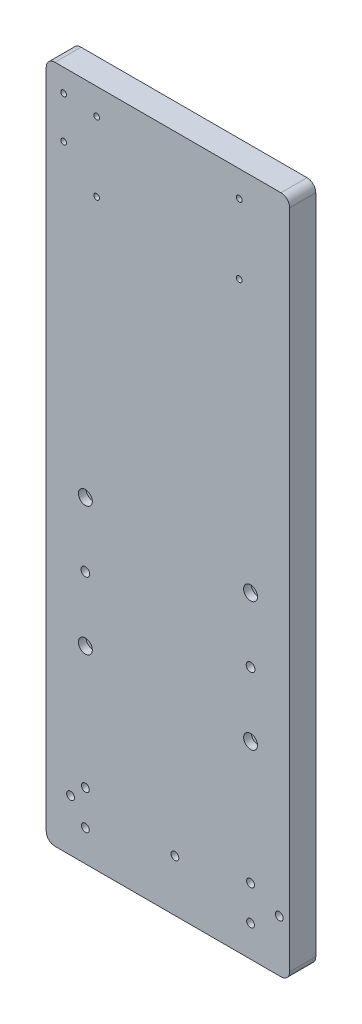
SolidWorks part; units mm, degrees
ref_plane "前视基准面" through (0, 0, 0) normal (0, 0, 1) x (1, 0, 0)
ref_plane "上视基准面" through (0, 0, 0) normal (0, 1, 0) x (1, 0, 0)
ref_plane "右视基准面" through (0, 0, 0) normal (1, 0, 0) x (0, 0, -1)
sketch "草图1" plane through (0, 0, 0) normal (0, 0, 1) x (1, 0, 0)
  line L1 (-70, 195.25) -> (70, 195.25)
  line L2 (-70, 195.25) -> (-70, -195.25)
  line L3 (-70, -195.25) -> (70, -195.25)
  line L4 (70, 195.25) -> (70, -195.25)
  line L5 (-70, 195.25) -> (70, -195.25) construction
  line L6 (-70, -195.25) -> (70, 195.25) construction
  point P0 (0, 0)
  dimension "D1" = 140
  dimension "D2" = 390.5
extrude "凸台-拉伸1" add sketch "草图1" along normal blind 15
sketch "草图29" plane through (0, 0, 0) normal (0, 0, -1) x (-1, 0, 0)
  line L0 (0, 0) -> (-70, 0) construction
  line L1 (-7.5, 45) -> (7.5, 45)
  line L2 (-7.5, 45) -> (-7.5, -45)
  line L3 (-7.5, -45) -> (7.5, -45)
  line L4 (7.5, 45) -> (7.5, -45)
  line L5 (-70, 195.25) -> (70, 195.25) construction
  line L10 (-70, -195.25) -> (-70, 195.25) construction
  line L11 (0, 195.25) -> (0, 0) construction
  dimension "D2" = 90
  dimension "D4" = 15
extrude "凸台-拉伸6" [suppressed] add sketch "草图29" against normal blind 165
hole_wizard "M5 六角凹头螺钉的柱形沉头孔6" positions "草图30" profile "草图31" counterbore size "M4" standard "ISO" end condition through all
sketch "草图30" plane through (0, 0, 15) normal (0, 0, 1) x (1, 0, 0)
  circle A0 centre (47.5, -12.75) radius 2.1 construction
  circle A1 centre (-47.5, -12.75) radius 2.1 construction
  circle A2 centre (47.5, -86.75) radius 2.1 construction
  circle A3 centre (-47.5, -86.75) radius 2.1 construction
  point P0 (-47.5, -12.75)
  point P4 (-47.5, -86.75)
  point P6 (47.5, -12.75)
  point P10 (47.5, -86.75)
sketch "草图31" plane through (-47.5, -12.75, 15) normal (1, 0, 0) x (0, -1, 0)
  line L0 (0, 0) -> (0, 15)
  line L1 (0, 15) -> (2.25, 15)
  line L3 (2.25, 15) -> (2.25, 4.4)
  line L4 (2.25, 4.4) -> (4, 4.4)
  line L5 (4, 4.4) -> (4, 0)
  line L7 (4, 0) -> (0, 0)
  line L11 (0, -6.35) -> (0, 107.95) construction
  dimension "通孔孔直径" = 4.5
  dimension "通孔孔深度" = 15
  dimension "柱形沉头孔直径" = 8
  dimension "柱形沉头孔深度" = 4.4
hole_wizard "Ø5.0 (5) 直径孔1" positions "草图32" profile "草图33" hole size "Ø5.0" standard "ISO" end condition through all
sketch "草图32" plane through (0, 0, 15) normal (0, 0, 1) x (1, 0, 0)
  circle A0 centre (47.5, -49.75) radius 2.5 construction
  circle A1 centre (-47.5, -49.75) radius 2.5 construction
  point P0 (-47.5, -49.75)
  point P2 (47.5, -49.75)
sketch "草图33" plane through (-47.5, -49.75, 15) normal (1, 0, 0) x (0, -1, 0)
  line L0 (0, 0) -> (0, 15)
  line L1 (0, 15) -> (2.5, 15)
  line L2 (2.5, 15) -> (2.5, 0)
  line L5 (2.5, 0) -> (0, 0)
  line L11 (0, -6.35) -> (0, 107.95) construction
  dimension "通孔孔直径" = 5
  dimension "通孔孔深度" = 15
fillet "圆角1" radius 5 4 edges at (70, -195.25, 7.5) (70, 195.25, 7.5) (-70, -195.25, 7.5) (-70, 195.25, 7.5)
hole_wizard "M4 螺纹孔3" positions "草图38" profile "草图39" tap size "M4" standard "ISO" end condition through all
sketch "草图38" plane through (0, 0, 15) normal (0, 0, 1) x (1, 0, 0)
  point P0 (-41, 180.25)
  point P3 (41, 180.25)
  point P6 (41, 140.25)
  point P9 (-41, 140.25)
sketch "草图39" plane through (-41, 180.25, 15) normal (1, 0, 0) x (0, -1, 0)
  line L0 (0, 0) -> (0, 15)
  line L1 (0, 15) -> (1.65, 15)
  line L2 (1.65, 15) -> (1.65, 0)
  line L5 (1.65, 0) -> (0, 0)
  line L11 (0, -6.35) -> (0, 107.95) construction
  dimension "通孔螺纹孔钻头直径" = 3.3
  dimension "通孔螺纹孔钻头深度" = 15
cosmetic thread "孔螺蚊线8" parameters "D2"=4
cosmetic thread "孔螺蚊线9" parameters "D2"=4
cosmetic thread "孔螺蚊线23" parameters "D2"=4
cosmetic thread "孔螺蚊线24" parameters "D2"=4
hole_wizard "M4 六角凹头螺钉的柱形沉头孔1" positions "草图44" profile "草图45" counterbore size "M4" standard "ISO" end condition through all
sketch "草图44" plane through (0, 0, 0) normal (0, 0, -1) x (-1, 0, 0)
  circle A0 centre (47.5, -157.25) radius 1.65 construction
  circle A1 centre (47.5, -177.25) radius 1.65 construction
  circle A2 centre (-47.5, -157.25) radius 1.65 construction
  circle A3 centre (-47.5, -177.25) radius 1.65 construction
  point P0 (47.5, -157.25)
  point P2 (47.5, -177.25)
  point P4 (-47.5, -157.25)
  point P6 (-47.5, -177.25)
sketch "草图45" plane through (-47.5, -157.25, 0) normal (1, 0, 0) x (0, 1, 0)
  line L0 (0, 0) -> (0, 15)
  line L1 (0, 15) -> (2.25, 15)
  line L3 (2.25, 15) -> (2.25, 4.4)
  line L4 (2.25, 4.4) -> (4, 4.4)
  line L5 (4, 4.4) -> (4, 0)
  line L7 (4, 0) -> (0, 0)
  line L11 (0, -6.35) -> (0, 107.95) construction
  dimension "通孔孔直径" = 4.5
  dimension "通孔孔深度" = 15
  dimension "柱形沉头孔直径" = 8
  dimension "柱形沉头孔深度" = 4.4
hole_wizard "M4 螺纹孔6" positions "草图48" profile "草图50" tap size "M4" standard "ISO"
sketch "草图48" plane through (-70, 0, 0) normal (-1, 0, 0) x (0, 0, 1)
  line L0 (7.5, 195.25) -> (7.5, -195.25) construction
  line L1 (0, 195.25) -> (15, 195.25) construction
  line L2 (15, -195.25) -> (0, -195.25) construction
  point P0 (7.5, 185.25)
  point P2 (7.5, 170.25)
  point P4 (7.5, 155.25)
  dimension "D1" = 10
  dimension "D2" = 15
  dimension "D3" = 15
sketch "草图50" plane through (-70, 185.25, 7.5) normal (0, 1, 0) x (0, 0, 1)
  line L0 (0, 0) -> (0, 15.9914)
  line L1 (0, 15.9914) -> (1.65, 15)
  line L2 (1.65, 15) -> (1.65, 0)
  line L5 (1.65, 0) -> (0, 0)
  line L10 (0, 15.9914) -> (-1.65, 15) construction
  line L11 (0, -6.35) -> (0, 107.95) construction
  dimension "螺纹孔钻头直径" = 3.3
  dimension "螺纹孔钻头深度" = 15
  dimension "导头角度" = 118
cosmetic thread "孔螺蚊线18" parameters "D1"=15, "D2"=4
cosmetic thread "孔螺蚊线19" parameters "D1"=15, "D2"=4
cosmetic thread "孔螺蚊线20" parameters "D1"=15, "D2"=4
hole_wizard "M4 螺纹孔7" positions "草图51" profile "草图52" tap size "M4" standard "ISO" end condition through all
sketch "草图51" plane through (0, 0, 15) normal (0, 0, 1) x (1, 0, 0)
  line L0 (-60, 190.25) -> (-60, 150.25)
  arc A0 (-57.75, 188) -> (-62.25, 188) centre (-60, 188) ccw construction
  arc A1 (-62.25, 152.5) -> (-57.75, 152.5) centre (-60, 152.5) ccw construction
  point P0 (-60, 182.25)
  point P2 (-60, 158.25)
  dimension "D1" = 8
  dimension "D2" = 8
sketch "草图52" plane through (-60, 182.25, 15) normal (1, 0, 0) x (0, -1, 0)
  line L0 (0, 0) -> (0, 15)
  line L1 (0, 15) -> (1.65, 15)
  line L2 (1.65, 15) -> (1.65, 0)
  line L5 (1.65, 0) -> (0, 0)
  line L11 (0, -6.35) -> (0, 107.95) construction
  dimension "通孔螺纹孔钻头直径" = 3.3
  dimension "通孔螺纹孔钻头深度" = 15
cosmetic thread "孔螺蚊线21" parameters "D1"=15, "D2"=4
cosmetic thread "孔螺蚊线22" parameters "D1"=15, "D2"=4
hole_wizard "M4 六角凹头螺钉的柱形沉头孔2" positions "草图53" profile "草图54" counterbore size "M4" standard "ISO" end condition through all
sketch "草图53" plane through (0, 0, 0) normal (0, 0, -1) x (-1, 0, 0)
  circle A0 centre (56, -165.54) radius 1.65 construction
  circle A1 centre (-4, -165.54) radius 1.65 construction
  circle A2 centre (-64, -165.54) radius 1.65 construction
  circle A3 centre (-64, -225.54) radius 1.65 construction
  circle A4 centre (-4, -225.54) radius 1.65 construction
  circle A5 centre (56, -225.54) radius 1.65 construction
  point P0 (-64, -165.54)
  point P2 (-4, -165.54)
  point P4 (-64, -225.54)
  point P6 (-4, -225.54)
  point P8 (56, -165.54)
  point P10 (56, -225.54)
sketch "草图54" plane through (64, -165.54, 0) normal (1, 0, 0) x (0, 1, 0)
  line L0 (0, 0) -> (0, 15)
  line L1 (0, 15) -> (2.25, 15)
  line L3 (2.25, 15) -> (2.25, 4.4)
  line L4 (2.25, 4.4) -> (4, 4.4)
  line L5 (4, 4.4) -> (4, 0)
  line L7 (4, 0) -> (0, 0)
  line L11 (0, -6.35) -> (0, 107.95) construction
  dimension "通孔孔直径" = 4.5
  dimension "通孔孔深度" = 15
  dimension "柱形沉头孔直径" = 8
  dimension "柱形沉头孔深度" = 4.4
